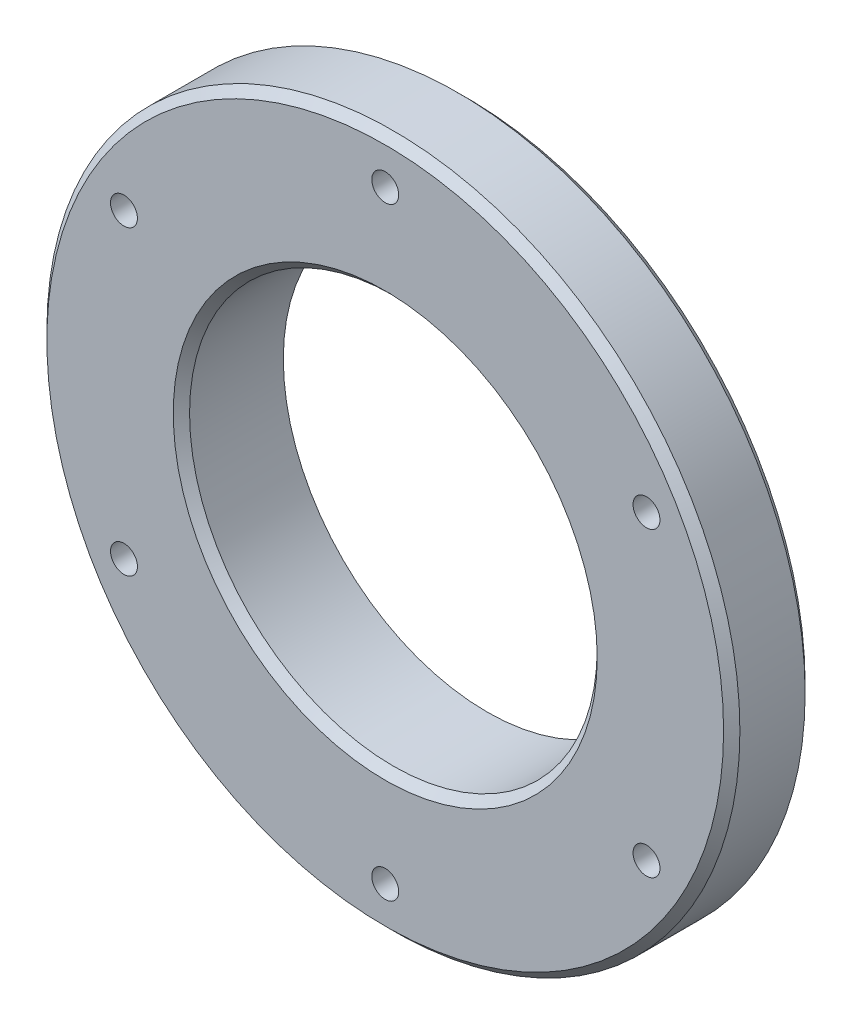
from build123d import *

# Parameters (mm, degrees)
SKETCH1_R                 = 42.5
SKETCH1_R_2               = 25
BOSS_EXTRUDE1_DEPTH       = 10
CHAMFER1_SIZE             = 1
M4X0_7_TAPPED_HOLE1_D     = 3.3
M4X0_7_TAPPED_HOLE1_DEPTH = 6
M4X0_7_TAPPED_HOLE1_TIP   = 0.991420021
BOSS_EXTRUDE2_START       = 2.5
SKETCH5_R                 = 35
SKETCH5_R_2               = 25
BOSS_EXTRUDE2_DEPTH       = 2.5


with BuildPart() as part:
    # Sketch1 → Boss-Extrude1 (new body)
    with BuildSketch(Plane.XY):
        Circle(SKETCH1_R)
        Circle(SKETCH1_R_2, mode=Mode.SUBTRACT)
    extrude(amount=BOSS_EXTRUDE1_DEPTH)

    # Chamfer1
    chamfer1_edges = [part.edges().sort_by_distance(p)[0] for p in [
        (-42.5, 0, 0),
        (-42.5, 0, 10),
        (-25, 0, 10),
    ]]
    chamfer(chamfer1_edges, length=CHAMFER1_SIZE)

    # M4x0.7 Tapped Hole1
    with Locations(Plane(origin=(0, 37, 10), x_dir=(1, 0, 0), z_dir=(0, 0, 1))):
        with Locations((0, 0), (32.04343994, -18.499133975), (32.04443994, -55.499133975), (0.002, -74), (-32.04143994, -55.500866025), (-32.04243994, -18.500866025)):
            Hole(M4X0_7_TAPPED_HOLE1_D / 2, depth=M4X0_7_TAPPED_HOLE1_DEPTH)
            with Locations((0, 0, -(M4X0_7_TAPPED_HOLE1_DEPTH + M4X0_7_TAPPED_HOLE1_TIP / 2))):  # 118° drill point
                Cone(0, M4X0_7_TAPPED_HOLE1_D / 2, M4X0_7_TAPPED_HOLE1_TIP, mode=Mode.SUBTRACT)

    # Sketch5 → Boss-Extrude2 (add)
    with BuildSketch(Plane(origin=(0, 0, 0), x_dir=(-1, 0, 0), z_dir=(0, 0, -1)).offset(BOSS_EXTRUDE2_START)):
        with Locations(Location((0, 0, 0), (0, 0, 180))):
            Circle(SKETCH5_R)
        Circle(SKETCH5_R_2, mode=Mode.SUBTRACT)
    extrude(amount=-BOSS_EXTRUDE2_DEPTH)


solid = part.part
